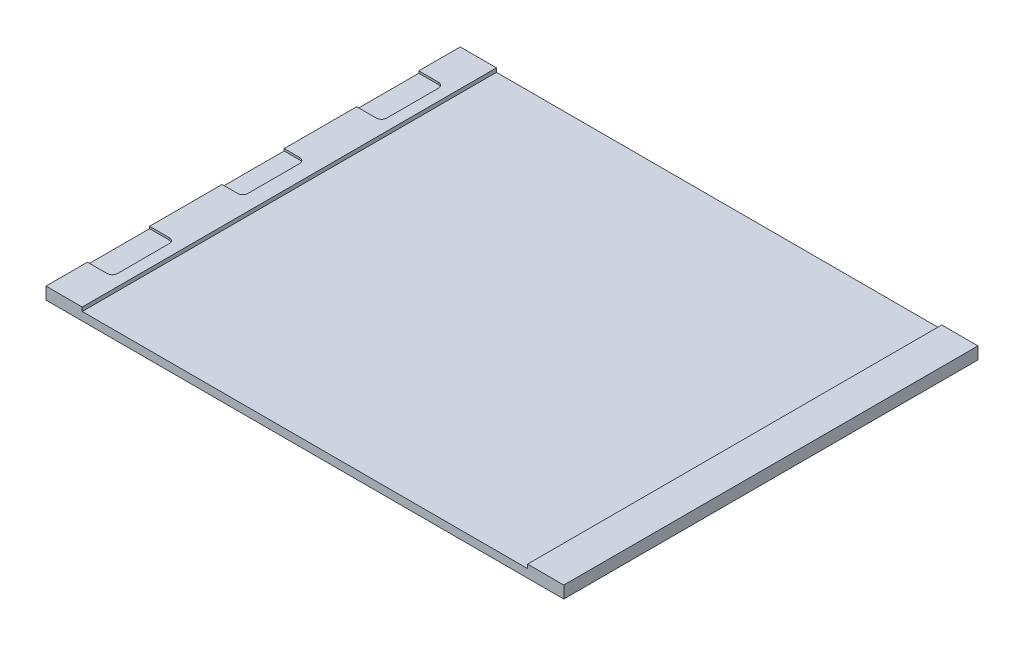
SolidWorks part; units mm, degrees
material "玻璃"
ref_plane "Front" through (0, 0, 0) normal (0, 0, 1) x (1, 0, 0)
ref_plane "Top" through (0, 0, 0) normal (0, 1, 0) x (1, 0, 0)
ref_plane "Right" through (0, 0, 0) normal (1, 0, 0) x (0, 0, -1)
sketch "Sketch1" plane through (0, 0, 0) normal (0, 0, 1) x (1, 0, 0)
  line L1 (0, 0) -> (500, 0)
  line L2 (0, 0) -> (0, 24)
  line L3 (0, 24) -> (500, 24)
  line L4 (500, 0) -> (500, 24)
  dimension "D1" = 500
  dimension "D2" = 24
extrude "Boss-Extrude1" add sketch "Sketch1" against normal blind 400
sketch "Sketch2" plane through (0, 0, 0) normal (0, 0, 1) x (1, 0, 0)
  line L0 (0, 12) -> (35, 12) construction
  line L1 (35, 16) -> (465, 16)
  line L2 (35, 16) -> (35, 8)
  line L3 (35, 8) -> (465, 8)
  line L4 (465, 16) -> (465, 8)
  line L5 (0, 24) -> (0, 0) construction
  line L6 (250, 24) -> (250, 16) construction
  line L7 (500, 24) -> (0, 24) construction
  dimension "D1" = 430
  dimension "D2" = 8
extrude "Cut-Extrude1" cut sketch "Sketch2" against normal through all
sketch "Sketch3" plane through (0, 0, 0) normal (0, 0, 1) x (1, 0, 0)
  line L0 (250, 16) -> (250, 8) construction
  line L1 (465, 16) -> (35, 16) construction
  line L2 (35, 8) -> (465, 8) construction
  line L4 (-22.4785, 12.25) -> (522.4785, 12.25)
  line L5 (-22.4785, 12.25) -> (-22.4785, 11.75)
  line L6 (-22.4785, 11.75) -> (522.4785, 11.75)
  line L7 (522.4785, 12.25) -> (522.4785, 11.75)
  line L8 (-22.4785, 12.25) -> (522.4785, 11.75) construction
  line L9 (-22.4785, 11.75) -> (522.4785, 12.25) construction
  point P6 (250, 12)
  dimension "D1" = 0.5
extrude "Cut-Extrude2" cut sketch "Sketch3" against normal through all
sketch "Sketch4" plane through (0, 0, 0) normal (-1, 0, 0) x (0, 0, 1)
  line L0 (-400, 24) -> (0, 24) construction
  line L1 (-370, 24) -> (-320, 24)
  line L2 (-370, 24) -> (-370, 0)
  line L3 (-370, 0) -> (-320, 0)
  line L4 (-320, 24) -> (-320, 0)
  line L5 (-400, 0) -> (0, 0) construction
  line L6 (-400, 24) -> (-400, 12.25) construction
  line L7 (-200, 24) -> (-200, 0) construction
  line L8 (-80, 24) -> (-80, 0)
  line L9 (-30, 0) -> (-80, 0)
  line L10 (-30, 24) -> (-30, 0)
  line L11 (-30, 24) -> (-80, 24)
  dimension "D1" = 30
  dimension "D2" = 50
sketch "Sketch12" plane through (0, 0, 0) normal (0, 0, 1) x (1, 0, 0)
  line L0 (0, 0) -> (500, 0) construction
  line L1 (-19.3284, 51.3288) -> (549.6795, 51.3288)
  line L2 (-19.3284, 51.3288) -> (-19.3284, 12)
  line L3 (-19.3284, 12) -> (549.6795, 12)
  line L4 (549.6795, 51.3288) -> (549.6795, 12)
  dimension "D1" = 12
extrude "Cut-Extrude3" cut sketch "Sketch12" against normal through all
sketch "Sketch16" plane through (0, 11.75, 0) normal (0, 1, 0) x (1, 0, 0)
  line L0 (0, 400) -> (0, 0) construction
  line L1 (0, 360) -> (24, 360)
  line L2 (0, 360) -> (0, 300)
  line L3 (0, 300) -> (24, 300)
  line L4 (24, 360) -> (24, 300)
  line L5 (0, 200) -> (21.3837, 200) construction
  line L6 (24, 40) -> (24, 100)
  line L7 (0, 100) -> (24, 100)
  line L8 (0, 40) -> (0, 100)
  line L9 (0, 40) -> (24, 40)
  line L11 (20, 230) -> (0, 230)
  line L12 (20, 230) -> (20, 170)
  line L13 (20, 170) -> (0, 170)
  line L14 (0, 230) -> (0, 170)
  dimension "D1" = 24
  dimension "D2" = 60
  dimension "D3" = 200
  dimension "D4" = 60
  dimension "D5" = 20
extrude "Cut-Extrude4" cut sketch "Sketch16" against normal blind 2
fillet "Fillet1" radius 5 6 edges at (24, 10.75, -40) (24, 10.75, -100) (20, 10.75, -170) (20, 10.75, -230) (24, 10.75, -300) (24, 10.75, -360)
